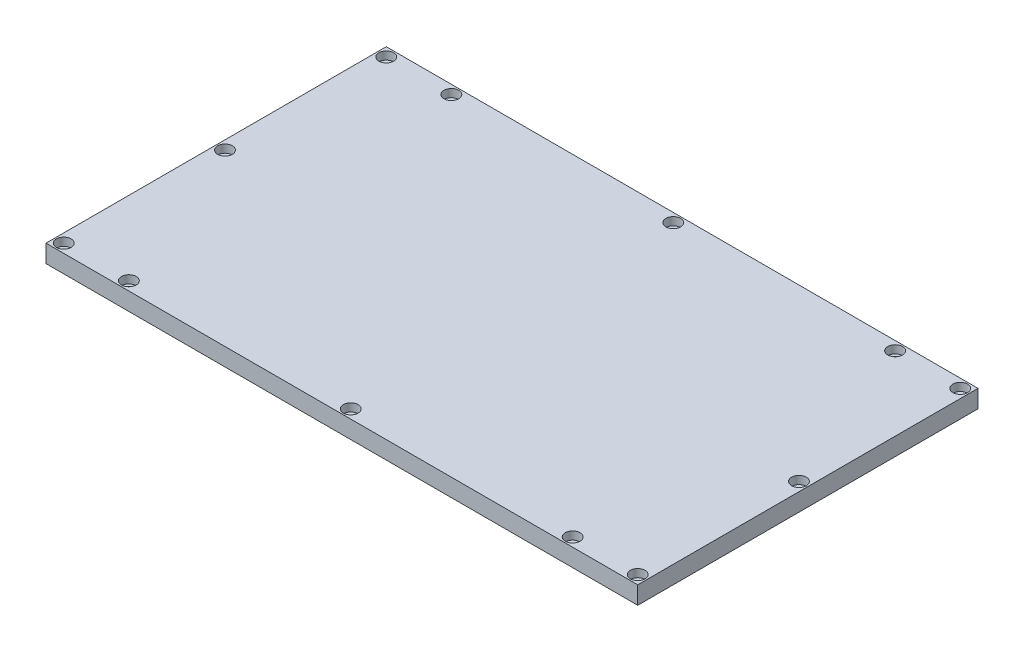
from build123d import *

# Parameters (mm, degrees)
SKETCH1_W                                           = 400
SKETCH1_H                                           = 230
BOSS_EXTRUDE1_DEPTH                                 = 12
CBORE_FOR_M5_HEX_SOCKET_HEAD_CAP_SCREW1_D           = 5.5
CBORE_FOR_M5_HEX_SOCKET_HEAD_CAP_SCREW1_DEPTH       = 24.5
CBORE_FOR_M5_HEX_SOCKET_HEAD_CAP_SCREW1_CBORE_D     = 10
CBORE_FOR_M5_HEX_SOCKET_HEAD_CAP_SCREW1_CBORE_DEPTH = 5.4
CBORE_FOR_M5_HEX_SOCKET_HEAD_CAP_SCREW1_TIP         = 1.652366702


with BuildPart() as part:
    # Sketch1 → Boss-Extrude1 (new body)
    with BuildSketch(Plane(origin=(0, 0, 0), x_dir=(1, 0, 0), z_dir=(0, 1, 0))):
        Rectangle(SKETCH1_W, SKETCH1_H)
    extrude(amount=BOSS_EXTRUDE1_DEPTH)

    # CBORE for M5 Hex Socket Head Cap Screw1
    with Locations(Plane(origin=(0, 12, 0), x_dir=(1, 0, 0), z_dir=(0, 1, 0))):
        with Locations((-194, 109), (-150, 109), (150, 109), (194, 109), (194, 0), (194, -109), (150, -109), (-150, -109), (-194, -109), (-194, 0), (0, 109), (0, -109)):
            CounterBoreHole(CBORE_FOR_M5_HEX_SOCKET_HEAD_CAP_SCREW1_D / 2, CBORE_FOR_M5_HEX_SOCKET_HEAD_CAP_SCREW1_CBORE_D / 2, CBORE_FOR_M5_HEX_SOCKET_HEAD_CAP_SCREW1_CBORE_DEPTH, depth=CBORE_FOR_M5_HEX_SOCKET_HEAD_CAP_SCREW1_DEPTH)
            with Locations((0, 0, -(CBORE_FOR_M5_HEX_SOCKET_HEAD_CAP_SCREW1_DEPTH + CBORE_FOR_M5_HEX_SOCKET_HEAD_CAP_SCREW1_TIP / 2))):  # 118° drill point
                Cone(0, CBORE_FOR_M5_HEX_SOCKET_HEAD_CAP_SCREW1_D / 2, CBORE_FOR_M5_HEX_SOCKET_HEAD_CAP_SCREW1_TIP, mode=Mode.SUBTRACT)


solid = part.part
